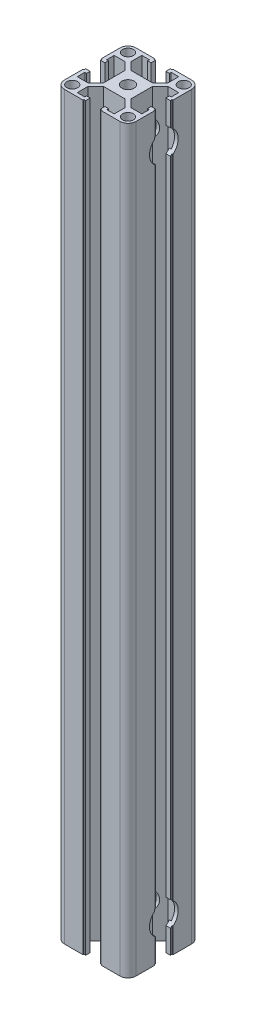
from build123d import *

# Parameters (mm, degrees)
SKETCH16_R                   = 3.4
SKETCH16_R_2                 = 3
MEMBER_1_DEPTH               = 413
HOLE_WIZARD_M8_1_D           = 9
HOLE_WIZARD_M8_1_CBORE_D     = 16
HOLE_WIZARD_M8_1_CBORE_DEPTH = 12.3


with BuildPart() as part:
    # Sketch16 → Member 1 (new body)
    with BuildSketch(Plane(origin=(0, 0, 0), x_dir=(-1, 0, 0), z_dir=(0, 1, 0))):
        with BuildLine():
            Line((-5.1, 20), (-5.1, 19.5))
            Line((-5.1, 19.5), (-4.1, 19.5))
            Line((-4.1, 19.5), (-4.1, 17))
            Line((-4.1, 17), (-6.1, 17))
            Line((-6.1, 17), (-6.1, 18))
            Line((-6.1, 18), (-10.3, 18))
            Line((-10.3, 18), (-10.3, 12))
            Line((-10.3, 12), (-6, 7.7))
            Line((-6, 7.7), (6, 7.7))
            Line((6, 7.7), (10.3, 12))
            Line((10.3, 12), (10.3, 18))
            Line((10.3, 18), (6.1, 18))
            Line((6.1, 18), (6.1, 17))
            Line((6.1, 17), (4.1, 17))
            Line((4.1, 17), (4.1, 19.5))
            Line((4.1, 19.5), (5.1, 19.5))
            Line((5.1, 19.5), (5.1, 20))
            Line((5.1, 20), (15.5, 20))
            ThreePointArc((15.5, 20), (18.681980515, 18.681980515), (20, 15.5))
            Line((20, 15.5), (20, 5.1))
            Line((20, 5.1), (19.5, 5.1))
            Line((19.5, 5.1), (19.5, 4.1))
            Line((19.5, 4.1), (17, 4.1))
            Line((17, 4.1), (17, 6.1))
            Line((17, 6.1), (18, 6.1))
            Line((18, 6.1), (18, 10.3))
            Line((18, 10.3), (12, 10.3))
            Line((12, 10.3), (7.7, 6))
            Line((7.7, 6), (7.7, -6))
            Line((7.7, -6), (12, -10.3))
            Line((12, -10.3), (18, -10.3))
            Line((18, -10.3), (18, -6.1))
            Line((18, -6.1), (17, -6.1))
            Line((17, -6.1), (17, -4.1))
            Line((17, -4.1), (19.5, -4.1))
            Line((19.5, -4.1), (19.5, -5.1))
            Line((19.5, -5.1), (20, -5.1))
            Line((20, -5.1), (20, -15.5))
            ThreePointArc((20, -15.5), (18.681980515, -18.681980515), (15.5, -20))
            Line((15.5, -20), (5.1, -20))
            Line((5.1, -20), (5.1, -19.5))
            Line((5.1, -19.5), (4.1, -19.5))
            Line((4.1, -19.5), (4.1, -17))
            Line((4.1, -17), (6.1, -17))
            Line((6.1, -17), (6.1, -18))
            Line((6.1, -18), (10.3, -18))
            Line((10.3, -18), (10.3, -12))
            Line((10.3, -12), (6, -7.7))
            Line((6, -7.7), (-6, -7.7))
            Line((-6, -7.7), (-10.3, -12))
            Line((-10.3, -12), (-10.3, -18))
            Line((-10.3, -18), (-6.1, -18))
            Line((-6.1, -18), (-6.1, -17))
            Line((-6.1, -17), (-4.1, -17))
            Line((-4.1, -17), (-4.1, -19.5))
            Line((-4.1, -19.5), (-5.1, -19.5))
            Line((-5.1, -19.5), (-5.1, -20))
            Line((-5.1, -20), (-15.5, -20))
            ThreePointArc((-15.5, -20), (-18.681980515, -18.681980515), (-20, -15.5))
            Line((-20, -15.5), (-20, -5.1))
            Line((-20, -5.1), (-19.5, -5.1))
            Line((-19.5, -5.1), (-19.5, -4.1))
            Line((-19.5, -4.1), (-17, -4.1))
            Line((-17, -4.1), (-17, -6.1))
            Line((-17, -6.1), (-18, -6.1))
            Line((-18, -6.1), (-18, -10.3))
            Line((-18, -10.3), (-12, -10.3))
            Line((-12, -10.3), (-7.7, -6))
            Line((-7.7, -6), (-7.7, 6))
            Line((-7.7, 6), (-12, 10.3))
            Line((-12, 10.3), (-18, 10.3))
            Line((-18, 10.3), (-18, 6.1))
            Line((-18, 6.1), (-17, 6.1))
            Line((-17, 6.1), (-17, 4.1))
            Line((-17, 4.1), (-19.5, 4.1))
            Line((-19.5, 4.1), (-19.5, 5.1))
            Line((-19.5, 5.1), (-20, 5.1))
            Line((-20, 5.1), (-20, 15.5))
            ThreePointArc((-20, 15.5), (-18.681980515, 18.681980515), (-15.5, 20))
            Line((-15.5, 20), (-5.1, 20))
        make_face()
        Circle(SKETCH16_R, mode=Mode.SUBTRACT)
        with Locations((-15.556349186, 15.556349186)):
            Circle(SKETCH16_R_2, mode=Mode.SUBTRACT)
        with Locations((15.556349186, 15.556349186)):
            Circle(SKETCH16_R_2, mode=Mode.SUBTRACT)
        with Locations((15.556349186, -15.556349186)):
            Circle(SKETCH16_R_2, mode=Mode.SUBTRACT)
        with Locations((-15.556349186, -15.556349186)):
            Circle(SKETCH16_R_2, mode=Mode.SUBTRACT)
    extrude(amount=MEMBER_1_DEPTH)

    # M8 六角凹头螺钉的柱形沉头孔1 (through all)
    with Locations(Plane(origin=(20, 0, 0), x_dir=(0, 0, -1), z_dir=(1, 0, 0))):
        with Locations((0, 20), (0, 393)):
            CounterBoreHole(HOLE_WIZARD_M8_1_D / 2, HOLE_WIZARD_M8_1_CBORE_D / 2, HOLE_WIZARD_M8_1_CBORE_DEPTH)


solid = part.part
